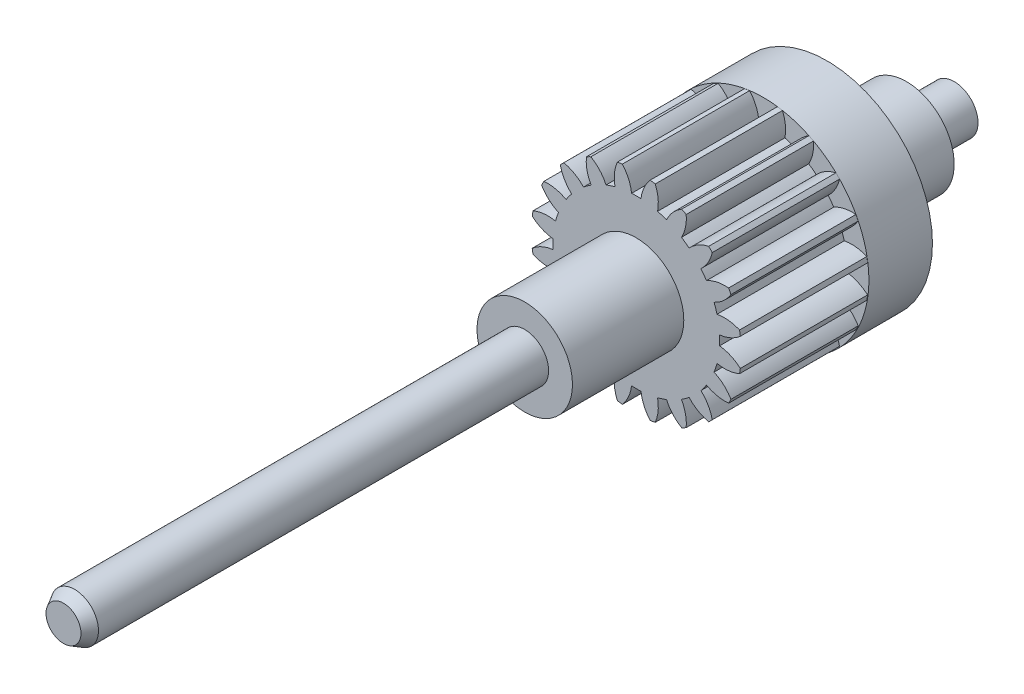
from build123d import *

# Parameters (mm, degrees)
BOSS_EXTRUDE_1_DEPTH = 4
SKETCH_3_R           = 3.317165214
BOSS_EXTRUDE_2_DEPTH = 2
SKETCH_4_R           = 1.5
BOSS_EXTRUDE_3_DEPTH = 2.5
BOSS_EXTRUDE_START   = 3.5
SKETCH_5_R           = 1.5
BOSS_EXTRUDE_4_DEPTH = 3.5
SKETCH_6_R           = 0.75
BOSS_EXTRUDE_5_DEPTH = 1.5
BOSS_EXTRUDE_START_2 = 14.5
SKETCH_7_R           = 0.75
BOSS_EXTRUDE_6_DEPTH = 14.5


with BuildPart() as part:
    # Sketch 1 → Boss-Extrude 1 (new body)
    with BuildSketch(Plane.XY):
        with BuildLine():
            ThreePointArc((-3.264884569, 0.453034732), (-2.961266903, 0.259072006), (-2.613758715, 0.163975816))
            ThreePointArc((-2.613758715, 0.163975816), (-2.617921702, 0.016225934), (-2.613758715, -0.131523948))
            ThreePointArc((-2.613758715, -0.131523948), (-2.961266903, -0.226620138), (-3.264884569, -0.420582864))
            ThreePointArc((-3.264884569, -0.420582864), (-3.253293226, -0.500007801), (-3.239773593, -0.579127326))
            ThreePointArc((-3.239773593, -0.579127326), (-2.891078254, -0.669773822), (-2.531191989, -0.652829737))
            ThreePointArc((-2.531191989, -0.652829737), (-2.489494001, -0.794634659), (-2.43987754, -0.933866714))
            ThreePointArc((-2.43987754, -0.933866714), (-2.740991128, -1.1316945), (-2.969810909, -1.409987033))
            ThreePointArc((-2.969810909, -1.409987033), (-2.934243232, -1.481942715), (-2.896936018, -1.553012059))
            ThreePointArc((-2.896936018, -1.553012059), (-2.537295737, -1.531469214), (-2.200259569, -1.40414346))
            ThreePointArc((-2.200259569, -1.40414346), (-2.116782295, -1.526122568), (-2.026569166, -1.643207791))
            ThreePointArc((-2.026569166, -1.643207791), (-2.251813058, -1.924402412), (-2.38343648, -2.25978354))
            ThreePointArc((-2.38343648, -2.25978354), (-2.32737408, -2.317226444), (-2.269931176, -2.373288844))
            ThreePointArc((-2.269931176, -2.373288844), (-1.934550048, -2.241665422), (-1.653355427, -2.01642153))
            ThreePointArc((-1.653355427, -2.01642153), (-1.536270204, -2.106634659), (-1.414291096, -2.190111933))
            ThreePointArc((-1.414291096, -2.190111933), (-1.54161685, -2.527148101), (-1.563159695, -2.886788382))
            ThreePointArc((-1.563159695, -2.886788382), (-1.492090351, -2.924095596), (-1.420134669, -2.959663273))
            ThreePointArc((-1.420134669, -2.959663273), (-1.141842136, -2.730843492), (-0.94401435, -2.429729904))
            ThreePointArc((-0.94401435, -2.429729904), (-0.804782295, -2.479346365), (-0.662977373, -2.521044353))
            ThreePointArc((-0.662977373, -2.521044353), (-0.679921458, -2.880930618), (-0.589274962, -3.229625956))
            ThreePointArc((-0.589274962, -3.229625956), (-0.510155437, -3.24314559), (-0.4307305, -3.254736932))
            ThreePointArc((-0.4307305, -3.254736932), (-0.236767774, -2.951119267), (-0.141671584, -2.603611078))
            ThreePointArc((-0.141671584, -2.603611078), (0.006078298, -2.607774066), (0.15382818, -2.603611078))
            ThreePointArc((0.15382818, -2.603611078), (0.24892437, -2.951119267), (0.442887096, -3.254736932))
            ThreePointArc((0.442887096, -3.254736932), (0.522312033, -3.24314559), (0.601431558, -3.229625956))
            ThreePointArc((0.601431558, -3.229625956), (0.692078054, -2.880930618), (0.675133969, -2.521044353))
            ThreePointArc((0.675133969, -2.521044353), (0.816938891, -2.479346365), (0.956170946, -2.429729904))
            ThreePointArc((0.956170946, -2.429729904), (1.153998732, -2.730843492), (1.432291265, -2.959663273))
            ThreePointArc((1.432291265, -2.959663273), (1.504246947, -2.924095596), (1.575316291, -2.886788382))
            ThreePointArc((1.575316291, -2.886788382), (1.553773446, -2.527148101), (1.426447692, -2.190111933))
            ThreePointArc((1.426447692, -2.190111933), (1.5484268, -2.106634659), (1.665512023, -2.01642153))
            ThreePointArc((1.665512023, -2.01642153), (1.946706645, -2.241665422), (2.282087772, -2.373288844))
            ThreePointArc((2.282087772, -2.373288844), (2.339530676, -2.317226444), (2.395593076, -2.25978354))
            ThreePointArc((2.395593076, -2.25978354), (2.263969654, -1.924402412), (2.038725762, -1.643207791))
            ThreePointArc((2.038725762, -1.643207791), (2.128938891, -1.526122568), (2.212416166, -1.40414346))
            ThreePointArc((2.212416166, -1.40414346), (2.549452333, -1.531469214), (2.909092614, -1.553012059))
            ThreePointArc((2.909092614, -1.553012059), (2.946399828, -1.481942715), (2.981967505, -1.409987033))
            ThreePointArc((2.981967505, -1.409987033), (2.753147724, -1.1316945), (2.452034136, -0.933866714))
            ThreePointArc((2.452034136, -0.933866714), (2.501650597, -0.794634659), (2.543348585, -0.652829737))
            ThreePointArc((2.543348585, -0.652829737), (2.90323485, -0.669773822), (3.251930189, -0.579127326))
            ThreePointArc((3.251930189, -0.579127326), (3.265449822, -0.500007801), (3.277041165, -0.420582864))
            ThreePointArc((3.277041165, -0.420582864), (2.973423499, -0.226620138), (2.625915311, -0.131523948))
            ThreePointArc((2.625915311, -0.131523948), (2.630078298, 0.016225934), (2.625915311, 0.163975816))
            ThreePointArc((2.625915311, 0.163975816), (2.973423499, 0.259072006), (3.277041165, 0.453034732))
            ThreePointArc((3.277041165, 0.453034732), (3.265449822, 0.532459669), (3.251930189, 0.611579194))
            ThreePointArc((3.251930189, 0.611579194), (2.90323485, 0.70222569), (2.543348585, 0.685281605))
            ThreePointArc((2.543348585, 0.685281605), (2.501650597, 0.827086527), (2.452034136, 0.966318582))
            ThreePointArc((2.452034136, 0.966318582), (2.753147724, 1.164146368), (2.981967505, 1.442438901))
            ThreePointArc((2.981967505, 1.442438901), (2.946399828, 1.514394583), (2.909092614, 1.585463927))
            ThreePointArc((2.909092614, 1.585463927), (2.549452333, 1.563921082), (2.212416166, 1.436595328))
            ThreePointArc((2.212416166, 1.436595328), (2.128938891, 1.558574436), (2.038725762, 1.675659659))
            ThreePointArc((2.038725762, 1.675659659), (2.263969654, 1.956854281), (2.395593076, 2.292235408))
            ThreePointArc((2.395593076, 2.292235408), (2.339530676, 2.349678312), (2.282087772, 2.405740712))
            ThreePointArc((2.282087772, 2.405740712), (1.946706645, 2.27411729), (1.665512023, 2.048873398))
            ThreePointArc((1.665512023, 2.048873398), (1.5484268, 2.139086527), (1.426447692, 2.222563802))
            ThreePointArc((1.426447692, 2.222563802), (1.553773446, 2.559599969), (1.575316291, 2.91924025))
            ThreePointArc((1.575316291, 2.91924025), (1.504246947, 2.956547464), (1.432291265, 2.992115141))
            ThreePointArc((1.432291265, 2.992115141), (1.153998732, 2.76329536), (0.956170946, 2.462181772))
            ThreePointArc((0.956170946, 2.462181772), (0.816938891, 2.511798233), (0.675133969, 2.553496221))
            ThreePointArc((0.675133969, 2.553496221), (0.692078054, 2.913382486), (0.601431558, 3.262077825))
            ThreePointArc((0.601431558, 3.262077825), (0.522312033, 3.275597458), (0.442887096, 3.287188801))
            ThreePointArc((0.442887096, 3.287188801), (0.24892437, 2.983571135), (0.15382818, 2.636062947))
            ThreePointArc((0.15382818, 2.636062947), (0.006078298, 2.640225934), (-0.141671584, 2.636062947))
            ThreePointArc((-0.141671584, 2.636062947), (-0.236767774, 2.983571135), (-0.4307305, 3.287188801))
            ThreePointArc((-0.4307305, 3.287188801), (-0.510155437, 3.275597458), (-0.589274962, 3.262077825))
            ThreePointArc((-0.589274962, 3.262077825), (-0.679921458, 2.913382486), (-0.662977373, 2.553496221))
            ThreePointArc((-0.662977373, 2.553496221), (-0.804782295, 2.511798233), (-0.94401435, 2.462181772))
            ThreePointArc((-0.94401435, 2.462181772), (-1.141842136, 2.76329536), (-1.420134669, 2.992115141))
            ThreePointArc((-1.420134669, 2.992115141), (-1.492090351, 2.956547464), (-1.563159695, 2.91924025))
            ThreePointArc((-1.563159695, 2.91924025), (-1.54161685, 2.559599969), (-1.414291096, 2.222563802))
            ThreePointArc((-1.414291096, 2.222563802), (-1.536270204, 2.139086527), (-1.653355427, 2.048873398))
            ThreePointArc((-1.653355427, 2.048873398), (-1.934550048, 2.27411729), (-2.269931176, 2.405740712))
            ThreePointArc((-2.269931176, 2.405740712), (-2.32737408, 2.349678312), (-2.38343648, 2.292235408))
            ThreePointArc((-2.38343648, 2.292235408), (-2.251813058, 1.956854281), (-2.026569166, 1.675659659))
            ThreePointArc((-2.026569166, 1.675659659), (-2.116782295, 1.558574436), (-2.200259569, 1.436595328))
            ThreePointArc((-2.200259569, 1.436595328), (-2.537295737, 1.563921082), (-2.896936018, 1.585463927))
            ThreePointArc((-2.896936018, 1.585463927), (-2.934243232, 1.514394583), (-2.969810909, 1.442438901))
            ThreePointArc((-2.969810909, 1.442438901), (-2.740991128, 1.164146368), (-2.43987754, 0.966318582))
            ThreePointArc((-2.43987754, 0.966318582), (-2.489494001, 0.827086527), (-2.531191989, 0.685281605))
            ThreePointArc((-2.531191989, 0.685281605), (-2.891078254, 0.70222569), (-3.239773593, 0.611579194))
            ThreePointArc((-3.239773593, 0.611579194), (-3.253293226, 0.532459669), (-3.264884569, 0.453034732))
        make_face()
    extrude(amount=BOSS_EXTRUDE_1_DEPTH)

    # Sketch 3 → Boss-Extrude 2 (add)
    with BuildSketch(Plane.XY):
        Circle(SKETCH_3_R)
    extrude(amount=-BOSS_EXTRUDE_2_DEPTH)

    # Sketch 4 → Boss-Extrude 3 (add)
    with BuildSketch(Plane(origin=(0, 0, -2), x_dir=(-1, 0, 0), z_dir=(0, 0, -1))):
        Circle(SKETCH_4_R)
    extrude(amount=BOSS_EXTRUDE_3_DEPTH)

    # Sketch 5 → Boss-Extrude 4 (add)
    with BuildSketch(Plane.XY.offset(4).offset(BOSS_EXTRUDE_START)):
        with Locations(Location((0, 0, 0), (0, 0, 180))):
            Circle(SKETCH_5_R)
    extrude(amount=-BOSS_EXTRUDE_4_DEPTH)

    # Sketch 6 → Boss-Extrude 5 (add)
    with BuildSketch(Plane(origin=(0, 0, -4.5), x_dir=(-1, 0, 0), z_dir=(0, 0, -1))):
        Circle(SKETCH_6_R)
    extrude(amount=BOSS_EXTRUDE_5_DEPTH)

    # Sketch 7 → Boss-Extrude 6 (add)
    with BuildSketch(Plane.XY.offset(7.5).offset(BOSS_EXTRUDE_START_2)):
        with Locations(Location((0, 0, 0), (0, 0, 180))):
            Circle(SKETCH_7_R)
    extrude(amount=-BOSS_EXTRUDE_6_DEPTH)

    # Sketch 9 → Cut-Revolve 1 (revolve, cut)
    with BuildSketch(Plane(origin=(0, 0, 0), x_dir=(1, 0, 0), z_dir=(0, 1, 0)), mode=Mode.PRIVATE) as cut_revolve_1_sk:
        Polygon((0.55, -22), (0.75, -22), (0.75, -21.65), align=None)
    revolve(cut_revolve_1_sk.sketch.rotate(Axis((0, 0, 22), (0, 0, -1)), 180), axis=Axis((0, 0, 22), (0, 0, -1)), mode=Mode.SUBTRACT)


solid = part.part
